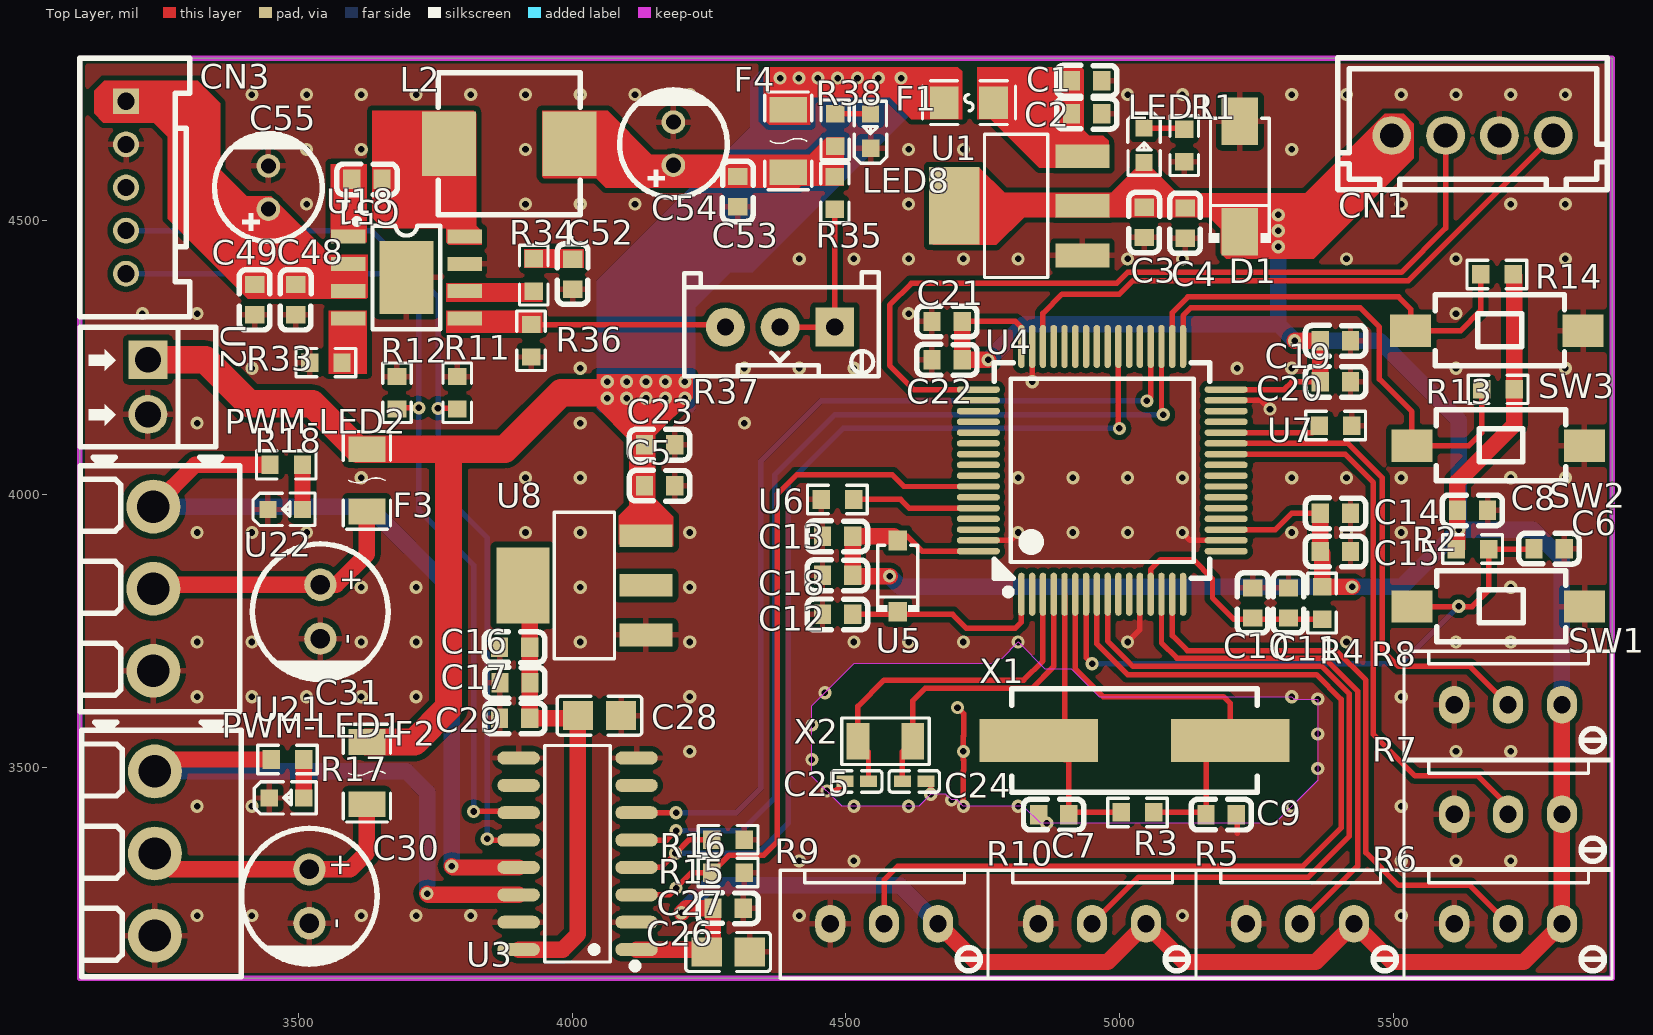
[diagram p0: Top Layer view]
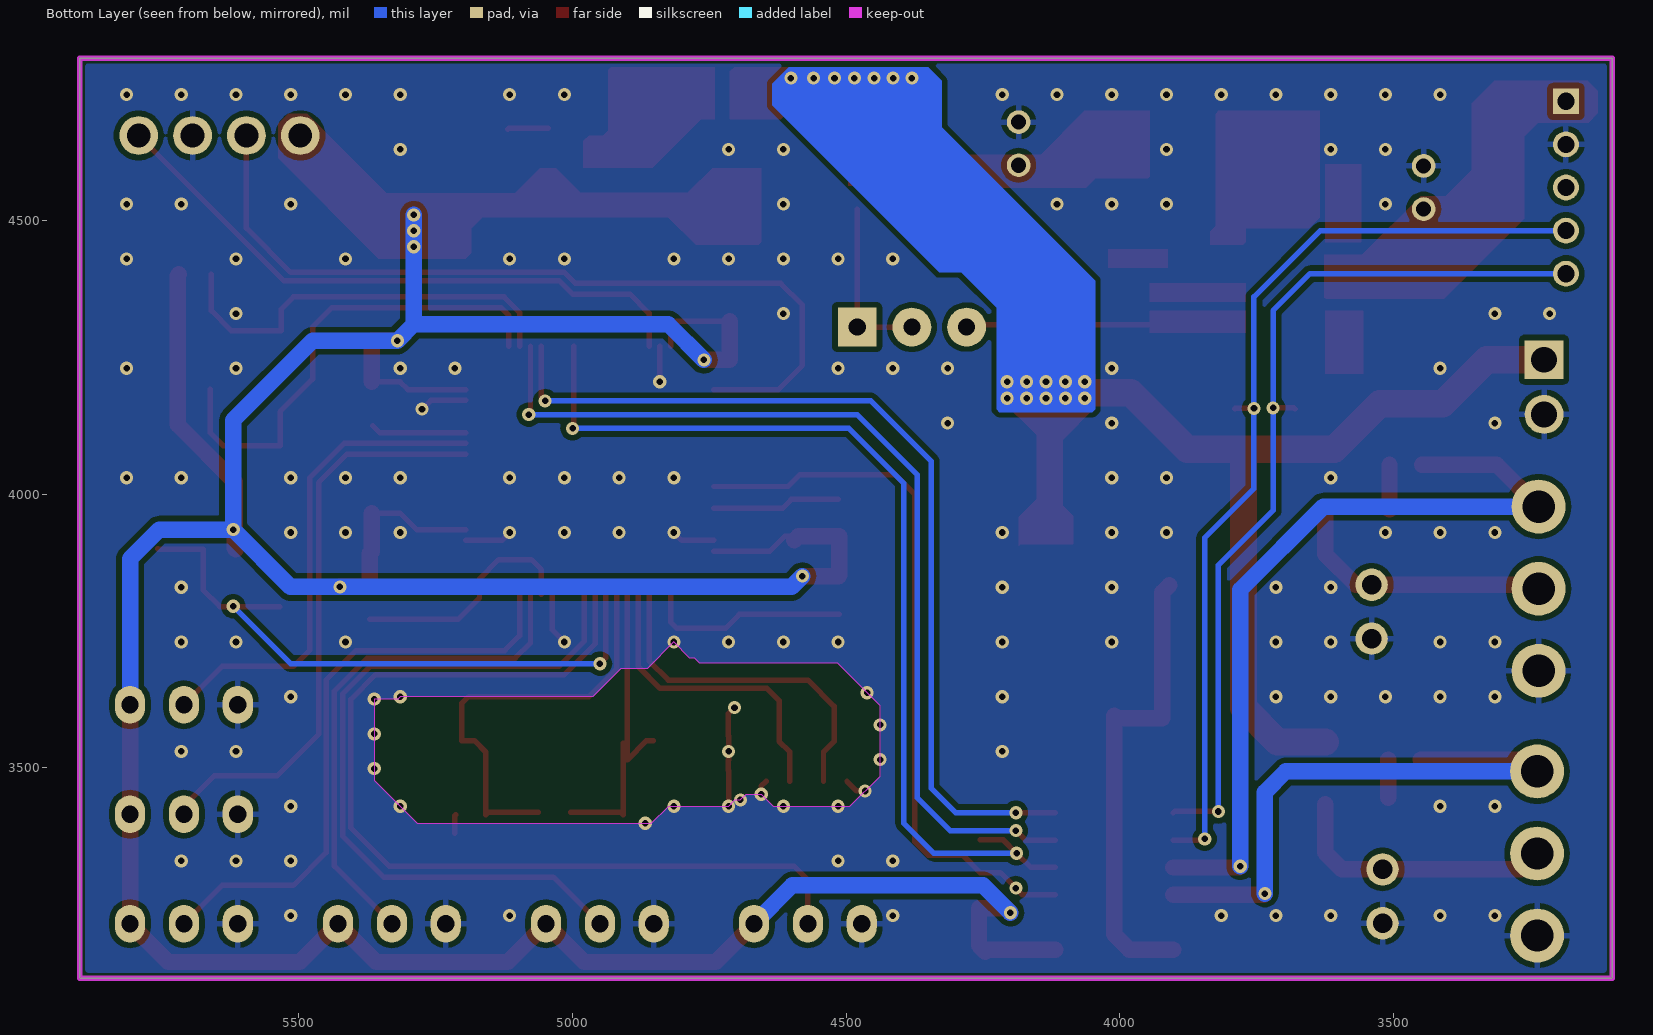
[diagram p1: Bottom Layer view, seen from below]
# Altium PCB MISC49876.pcbdoc
Units mil, origin at the board's own origin, x right, y up, seen from the top; angles counter-clockwise.
Board outline 2799.25 x 1680.67 mil, 2 copper layers (Top Layer, Bottom Layer), stack 62.206 mil thick; 90 components, 54 nets, 281 pads, 188 vias.

## Layer stack, top to bottom
Top Solder Mask Layer: solder mask 0.394, Dk 3.3
Top Layer: signal copper 1.379
Dielectric1: surface 59.449, FR4, Dk 4.5
Bottom Layer: signal copper 1.378
Bottom Solder Mask Layer: solder mask 0.394, Dk 3.3

## Board outline
3100.75,4796.22 3100.75,3115.55 5900,3115.55 5900,4796.22

## Design rules (kind name [scope] priority, off if disabled: settings)
BoardOutlineClearance copperThickness2oz_1 [All] p2 off: genericclearance=7.99 ignorepadtopadclearanceinfootprint=FALSE except(0: Arc-SplitContinuation Track-SplitContinuation SMDPad-SplitContinuation THPad-SplitContinuation Via-SplitContinuation Fill-SplitContinuation Region-SplitContinuation Poly-SplitContinuation Text-SplitContinuation Hole-SplitContinuation; 5.98: Arc-CutoutEdge SMDPad-CutoutEdge THPad-CutoutEdge Via-CutoutEdge Fill-CutoutEdge Region-CutoutEdge Text-CutoutEdge; 6.93: Hole-OutlineEdge Hole-CutoutEdge; 10: Poly-OutlineEdge Poly-CutoutEdge; 11.81: Arc-OutlineEdge Track-OutlineEdge SMDPad-OutlineEdge THPad-OutlineEdge Via-OutlineEdge Fill-OutlineEdge Region-OutlineEdge Text-OutlineEdge Track-CutoutEdge)
BoardOutlineClearance copperThickness1oz_1 [All] p4: genericclearance=4.02 ignorepadtopadclearanceinfootprint=FALSE except(0: Arc-SplitContinuation Track-SplitContinuation SMDPad-SplitContinuation THPad-SplitContinuation Via-SplitContinuation Fill-SplitContinuation Region-SplitContinuation Poly-SplitContinuation Text-SplitContinuation Hole-SplitContinuation; 6: SMDPad-CutoutEdge THPad-CutoutEdge Via-CutoutEdge Fill-CutoutEdge Region-CutoutEdge Text-CutoutEdge; 6.93: Hole-OutlineEdge Hole-CutoutEdge; 10: Poly-OutlineEdge Poly-CutoutEdge; 11.8: Arc-OutlineEdge Track-OutlineEdge SMDPad-OutlineEdge THPad-OutlineEdge Via-OutlineEdge Fill-OutlineEdge Region-OutlineEdge Text-OutlineEdge; 11.81: Arc-CutoutEdge Track-CutoutEdge)
Clearance copperThickness2oz [All] p1 off: gap=7.99 ignorepadtopadclearanceinfootprint=FALSE except(5.98: SMDPad-Track SMDPad-SMDPad THPad-Track SMDPad-THPad THPad-THPad Track-Via SMDPad-Via THPad-Via Via-Via Fill-Track Region-Track Fill-SMDPad Region-SMDPad Fill-THPad Region-THPad Fill-Via Region-Via Fill-Fill Fill-Region Region-Region Arc-Track Arc-SMDPad Arc-THPad Arc-Via Fill-Arc Region-Arc Arc-Arc Text-Track SMDPad-Text Text-THPad Text-Via Fill-Text Region-Text Arc-Text Text-Text; 6.93: Hole-Track Hole-SMDPad Hole-THPad Hole-Via Fill-Hole Region-Hole Hole-Arc Hole-Text; 10: Poly-Track Poly-SMDPad Poly-THPad Poly-Via Poly-Fill Poly-Region Poly-Poly Poly-Arc Poly-Text Poly-Hole)
Clearance copperThickness1oz [All] p3: gap=4.02 ignorepadtopadclearanceinfootprint=FALSE except(5.98: SMDPad-Track SMDPad-SMDPad THPad-Track SMDPad-THPad THPad-THPad Track-Via SMDPad-Via THPad-Via Via-Via Fill-Track Region-Track Fill-SMDPad Region-SMDPad Fill-THPad Region-THPad Fill-Via Region-Via Fill-Fill Fill-Region Region-Region; 6: Arc-Track Arc-SMDPad Arc-THPad Arc-Via Fill-Arc Region-Arc Arc-Arc Text-Track SMDPad-Text Text-THPad Text-Via Fill-Text Region-Text Arc-Text Text-Text; 6.93: Hole-Track Hole-SMDPad Hole-THPad Hole-Via Fill-Hole Region-Hole Hole-Arc Hole-Text; 10: Poly-Track Poly-SMDPad Poly-THPad Poly-Via Poly-Fill Poly-Region Poly-Poly Poly-Arc Poly-Text Poly-Hole)
DiffPairsRouting differentialPair [All] p1: maxlimit=6 minlimit=6 mostfreqgap=6 toplayer_minwidth=5 toplayer_prefwidth=10 toplayer_maxwidth=100 toplayer_mingap=6 toplayer_prefgap=6 toplayer_maxgap=6 bottomlayer_minwidth=5 bottomlayer_prefwidth=10 bottomlayer_maxwidth=100 bottomlayer_mingap=6 bottomlayer_prefgap=6 bottomlayer_maxgap=6 maxuncoupledlength=10
HoleToHoleClearance otherClearance [All] p1: gap=11.81 allowstackedmicrovias=TRUE
Length netLength [All] p1: minlimit=0 maxlimit=0
MatchedLengths netLengthTolerance [All] p1: tolerance=1000
PasteMaskExpansion pasteMaskExpansion [All] p1: expansion=0
PlaneConnect innerPlane [All] p1: planeconnectstyle=Relief reliefexpansion=20 reliefentries=4 reliefconductorwidth=10 reliefairgap=10
PolygonConnect copperRegion [(InNet('GND'))] p1: connectstyle=Relief reliefconductorwidth=10 reliefentries=4 polygonreliefangle="90 Angle" airgapwidth=10 via.connectstyle=Relief via.reliefconductorwidth=10 via.reliefentries=4 via.polygonreliefangle="90 Angle" via.airgapwidth=10
RoutingVias viaSize [All] p1: holewidth=12.01 width=24.02 viastyle="Through Hole" minholewidth=11.81 minwidth=19.68 maxholewidth=248.03 maxwidth=393.7
SolderMaskExpansion solderMaskExpansion [IsVia] p1: expansion=-1000 istentingtop=TRUE
SolderMaskExpansion solderMaskExpansion [All] p2: expansion=2 istentingtop=FALSE
Width copperThickness2oz_2 [All] p1 off: maxlimit=100 minlimit=8 preferedwidth=10
Width copperThickness1oz_2 [All] p2: maxlimit=100 minlimit=5 preferedwidth=10

## Components (designator, comment, footprint, x,y, rotation, side; value= is the part's Value field where it differs from the comment)
C1 "22uF" C0603 4940,4755 r180 top
C2 "100nF" C0603 4940,4695 r180 top
C3 "22uF" C0603 5045.23,4496.42 r90 top
C4 "100nF" C0603 5120,4495 r90 top
C5 "100nF" C0603 4160,4015 r0 top
C6 "100nF" C0603 5785,3900 r0 top
C7 "20pF" C0603 4880,3414.11 r0 top
C8 "100nF" C0603 5645,3970 r0 top
C9 "20pF" C0603 5185.77,3414.33 r180 top
C10 "100nF" C0603 5243.29,3800.87 r270 top
C11 "22uF" C0603 5308.85,3800.87 r270 top
C12 "100nF" C0603 4485,3780 r0 top
C13 "100nF" C0603 4485,3922.63 r0 top
C14 "100nF" C0603 5394.57,3964.89 r180 top
C15 "100nF" C0603 5394.57,3894.89 r180 top
C16 "22uF" C0603 3895,3720 r0 top
C17 "100nF" C0603 3895.61,3654.89 r0 top
C18 "100nF" C0603 4485,3851.32 r0 top
C19 "100nF" C0603 5394.57,4280 r180 top
C20 "100nF" C0603 5394.57,4205 r180 top
C21 "100nF" C0603 4685.01,4315.28 r0 top
C22 "100nF" C0603 4685.01,4245.02 r0 top
C23 "22uF" C0603 4160,4090 r0 top
C24 "9pF" C0402 4625,3475 r180 top
C25 "9pF" C0402 4520,3475 r0 top
C26 "10uF" C0805 4285,3163.34 r0 top
C27 "100nF" C0603 4285,3243.34 r180 top
C28 "10uF" C0805 4050,3595 r180 top
C29 "100nF" C0603 3895,3590 r180 top
C30 "1000uF" CAP-TH_BD6.3-P2.50-D0.5-FD 3520,3265 r270 top
C31 "1000uF" CAP-TH_BD6.3-P2.50-D0.5-FD 3540,3785 r270 top
C48 "100nF" C0603 3495,4355 r90 top
C49 "4.7uF" C0603 3420,4355 r90 top
C51 "100nF" C0603 3625,4575 r180 top
C52 "4.7nF" C0603 4000.83,4401.52 r270 top
C53 "47uF" C0603 4302.56,4552.56 r270 top
C54 "100uF" CAP-TH_BD5.0-P2.00-D0.5-FD 4185,4640 r90 top
C55 "100uF" CAP-TH_BD5.0-P2.00-D0.5-FD 3445,4560 r90 top
CN1 "HX25003-4A" CONN-TH_4P-P2.50_HX25003-4A 5645,4655 r180 top
CN3 "ZX-HY2.0-5PZZ" CONN-TH_5P-P2.00_ZX-HY2.0-5PZZ 3185,4560 r90 top
D1 "SS14" SMA_L4.2-W2.6-LS5.3-RD 5220,4580 r90 top
F1 "PICOSMDC050S-2" F0805 4725,4715 r0 top
F2 "JK-nSMD050-30" F1206 3625,3490 r90 top
F3 "JK-nSMD050-30" F1206 3625,4025 r90 top
F4 "SMD1206-050-16" F1206 4395,4645 r90 top
L2 "4.7uH" "0630 TPC 7*7*3" 3885,4640 r0 top
LED1 "" LED_0603 5045,4635 r270 top
LED8 "" LED_0603 4545,4665 r90 top
PWM-LED1 "" LED_0603 3480,3445 r0 top
PWM-LED2 "" LED_0603 3477.71,3972.13 r0 top
R1 "1kΩ" R0603 5118.46,4636.6 r90 top
R2 "10kΩ" R0603 5645.15,3899.36 r0 top
R3 "1MΩ" R0603 5032.88,3418.27 r0 top
R4 "10Ω" R0603 5370.26,3800.57 r270 top
R5 "5kΩ" RES-ADJ-TH_3296W-1-203 5330,3215 r0 top
R6 "5kΩ" RES-ADJ-TH_3296W-1-203 5710,3215 r0 top
R7 "5kΩ" RES-ADJ-TH_3296W-1-203 5710,3415 r0 top
R8 "5kΩ" RES-ADJ-TH_3296W-1-203 5710,3615 r0 top
R9 "5kΩ" RES-ADJ-TH_3296W-1-203 4570,3215 r0 top
R10 "5kΩ" RES-ADJ-TH_3296W-1-203 4950,3215 r0 top
R11 "10kΩ" R0603 3790,4185 r270 top
R12 "10kΩ" R0603 3680,4185 r270 top
R13 "10kΩ" R0603 5691.77,4191.18 r180 top
R14 "10kΩ" R0603 5689.56,4401.18 r180 top
R15 "10kΩ" R0603 4285,3308.34 r180 top
R16 "10kΩ" R0603 4285,3368.34 r180 top
R17 "1kΩ" R0603 3480,3515 r180 top
R18 "1kΩ" R0603 3477.71,4053.27 r180 top
R33 "200K" R0603 3550,4240 r0 top
R34 "20K" R0603 3930,4400 r90 top
R35 "27k" R0603 4480,4550 r90 top
R36 "8.2K" R0603 3925,4280 r90 top
R37 "50K" RESPOT3296 4380,4305 r180 top
R38 "1k" R0603 4480.53,4665.27 r270 top
SW1 "TS-1101-C-W" SW-SMD_L6.0-W3.3-LS8.0 5692.25,3794.36 r180 top
SW2 "TS-1101-C-W" SW-SMD_L6.0-W3.3-LS8.0 5691.77,4088.23 r180 top
SW3 "TS-1101-C-W" SW-SMD_L6.0-W3.3-LS8.0 5689.56,4298.23 r180 top
U1 "AMS1117-3.3" SOT-223-3_L6.5-W3.4-P2.30-LS7.0-BR 4815.23,4526.42 r0 top
U2 "DB125-2.54-2P-GN-S" CONN-TH_DB125-2.54-2P-GN 3225,4195.4 r270 top
U3 "π142U31" SOIC-16_L9.9-W3.9-P1.27-LS6.0-BL 4009.95,3342.69 r90 top
U4 "STM32F103RET6" LQFP-64_L10.0-W10.0-P0.50-LS12.0-BL 4968.51,4043.25 r0 top
U5 "IN4148 SMD diode" SOD-123_L2.7-W1.7-LS3.8-RD 4595,3850 r90 top
U6 "100k" R0603 4484.69,3990 r180 top
U7 "100k" R0603 5395,4125 r180 top
U8 "AMS1117-5.0" SOT-223_L6.5-W3.5-P2.30-LS7.0-BR 4022.43,3833.02 r0 top
U18 "SCT2450" SOP-8E 3697.19,4395.61 r0 top
U21 "DB125-3.81-3P-GN-S" CONN-TH_3P-P3.81_L7.4-W11.4 3237.71,3343.27 r270 top
U22 "DB125-3.81-3P-GN-S" CONN-TH_3P-P3.81_L7.4-W11.4 3235,3827.01 r270 top
X1 "8MHz" CRYSTAL-SMD_L11.5-W4.8-LS12.7 5027.4,3549.33 r0 top
X2 "32.768kHz" OSC-SMD_L3.2-W1.5 4572.4,3548.25 r0 top

## Footprints (in the part's own frame and the unit in brackets; to place one, negate y for a bottom-side part, rotate by r counter-clockwise, add the part's x,y. Pads: shape width x height; smd on the part's side, far side on the other; paste and mask are expansions set on the pad)
"0630 TPC 7*7*3" [mm]
  rect 2.5x3 smd: 1(-2.8,0) 2(2.8,0)
  silkscreen extent -3.3,-3.3 3.3,3.3
C0402 [mm]
  rect 0.79x0.54 smd paste-100 mask+0.051: 1(-0.545,0) 2(0.545,0)
  silkscreen extent -1.17,-0.5 1.17,0.5
C0603 [mm]
  rect 0.8x0.9 smd: 1(-0.7,0) 2(0.7,0)
  silkscreen extent -1.41,-0.71 1.39,0.72
C0805 [mm]
  rect 1.41x1.35 smd paste-100 mask+0.051: 1(-1,0) 2(1,0)
  silkscreen extent -1.96,-0.9 1.96,0.9
CAP-TH_BD5.0-P2.00-D0.5-FD [mm]
  round 1.1 hole 0.7 paste+0 mask+0.05: 1(-1,0) 2(1,0)
  silkscreen extent -2.5,-2.5 2.5,2.5
CAP-TH_BD6.3-P2.50-D0.5-FD [mm]
  round 1.5 hole 0.9 paste+0 mask+0.05: 1(-1.25,0) 2(1.25,0)
  silkscreen extent -3.15,-3.15 3.21,3.15
CONN-TH_3P-P3.81_L7.4-W11.4 [mm]
  round 2.5 hole 1.5: 1(-3.81,0) 2(0,0) 3(3.81,0)
  silkscreen extent -6.1,-3.4 5.71,4
CONN-TH_4P-P2.50_HX25003-4A [mm]
  round 1.8 hole 1.1: 1(-3.75,0) 2(-1.25,0) 3(1.25,0) 4(3.75,0)
  silkscreen extent -6.25,-3.6 6.25,2.51
CONN-TH_5P-P2.00_ZX-HY2.0-5PZZ [mm]
  rect 1.2x1.2 hole 0.8: 1(4,0)
  round 1.2 hole 0.8: 2(2,0) 3(0,0) 4(-2,0) 5(-4,0)
  silkscreen extent -6,-2.96 6,2.14
CONN-TH_DB125-2.54-2P-GN [mm]
  rect 1.8x1.8 hole 1.2: 1(-1.27,0)
  round 1.8 hole 1.2: 2(1.27,0)
  silkscreen extent -2.78,-3.14 2.78,3.14
CRYSTAL-SMD_L11.5-W4.8-LS12.7 [mm]
  rect 5.5x2 smd: 1(-4.45,0) 2(4.45,0)
  silkscreen extent -5.7,-2.4 5.7,2.4
F0805 [mm]
  rect 1.335x1.5 smd paste-100 mask+0.051: 1(-1.142,0) 2(1.142,0)
  silkscreen extent -2.16,-1.02 2.16,1.02
F1206 [mm]
  rect 1.19x1.728 smd: 1(-1.445,0) 2(1.445,0)
  silkscreen extent -2.27,-1.09 2.27,1.09
LED_0603 [mil]
  rect 31.5x31.5 smd paste+0 mask+2: 1(-33.5,-0.4) 2(29.5,-0.2)
  silkscreen extent -61,-30 53,30
LQFP-64_L10.0-W10.0-P0.50-LS12.0-BL [mm]
  oval 0.3x2 smd: 1(-3.75,-5.75) 2(-3.25,-5.75) 3(-2.75,-5.75) 4(-2.25,-5.75) 5(-1.75,-5.75) 6(-1.25,-5.75) 7(-0.75,-5.75) 8(-0.25,-5.75) 9(0.25,-5.75) 10(0.75,-5.75) 11(1.25,-5.75) 12(1.75,-5.75) 13(2.25,-5.75) 14(2.75,-5.75) 15(3.25,-5.75) 16(3.75,-5.75) 33(3.75,5.75) 34(3.25,5.75) 35(2.75,5.75) 36(2.25,5.75) 37(1.75,5.75) 38(1.25,5.75) 39(0.75,5.75) 40(0.25,5.75) 41(-0.25,5.75) 42(-0.75,5.75) 43(-1.25,5.75) 44(-1.75,5.75) 45(-2.25,5.75) 46(-2.75,5.75) 47(-3.25,5.75) 48(-3.75,5.75)
  oval 2x0.3 smd: 17(5.75,-3.75) 18(5.75,-3.25) 19(5.75,-2.75) 20(5.75,-2.25) 21(5.75,-1.75) 22(5.75,-1.25) 23(5.75,-0.75) 24(5.75,-0.25) 25(5.75,0.25) 26(5.75,0.75) 27(5.75,1.25) 28(5.75,1.75) 29(5.75,2.25) 30(5.75,2.75) 31(5.75,3.25) 32(5.75,3.75) 49(-5.75,3.75) 50(-5.75,3.25) 51(-5.75,2.75) 52(-5.75,2.25) 53(-5.75,1.75) 54(-5.75,1.25) 55(-5.75,0.75) 56(-5.75,0.25) 57(-5.75,-0.25) 58(-5.75,-0.75) 59(-5.75,-1.25) 60(-5.75,-1.75) 61(-5.75,-2.25) 62(-5.75,-2.75) 63(-5.75,-3.25) 64(-5.75,-3.75)
  silkscreen extent -5,-5.79 5,5
OSC-SMD_L3.2-W1.5 [mm]
  rect 1.05x1.7 smd: 1(-1.275,0) 2(1.275,0)
  silkscreen extent -2.03,-1.08 2.03,1.08
R0603 [mil]
  rect 31.75x34.02 smd paste-3937.01 mask+2: 1(-29.66,0) 2(29.66,0)
  silkscreen extent -55,-26 55,26
RES-ADJ-TH_3296W-1-203 [mm]
  oval 1.4x1.75 hole 0.8: 1(-2.5,0) 2(0,0) 3(2.5,0)
  silkscreen extent -4.83,-2.53 4.83,2.48
RESPOT3296 [mm]
  rect 1.8x1.8 hole 0.8: 1(-2.54,0)
  round 1.8 hole 0.8: 2(2.54,0) ADJ(0,0)
  silkscreen extent -4.57,-2.54 4.44,2.29
SMA_L4.2-W2.6-LS5.3-RD [mm]
  rect 2.2x1.7 smd: 1(-2.565,0) 2(2.565,0)
  silkscreen extent -3.08,-1.44 2.7,1.44
SOD-123_L2.7-W1.7-LS3.8-RD [mm]
  rect 0.91x0.84 smd: 1(-1.655,0) 2(1.655,0)
  silkscreen extent -1.65,-1 1.43,1
SOIC-16_L9.9-W3.9-P1.27-LS6.0-BL [mil]
  oval 23.7x77.6 smd: 1(-175,-107.7) 2(-125,-107.7) 3(-75,-107.7) 4(-25,-107.7) 5(25,-107.7) 6(75,-107.7) 7(125,-107.7) 8(175,-107.7) 9(175,107.7) 10(125,107.7) 11(75,107.7) 12(25,107.7) 13(-25,107.7) 14(-75,107.7) 15(-125,107.7) 16(-175,107.7)
  silkscreen extent -211,-111 198,60
SOP-8E [mm]
  rect 2.5x3.4 smd: 0(0,0)
  rect 1.6x0.65 smd: 1(-2.7,1.905) 2(-2.7,0.635) 3(-2.7,-0.635) 4(-2.7,-1.905) 5(2.7,-1.905) 6(2.7,-0.635) 7(2.7,0.635) 8(2.7,1.905)
  silkscreen extent -2.42,-2.4 1.58,2.72
SOT-223-3_L6.5-W3.4-P2.30-LS7.0-BR [mm]
  rect 2.5x1.1 smd: 1(2.97,-2.3) 2(2.97,0) 3(2.97,2.3)
  rect 2.34x3.6 smd: 4(-2.97,0)
  silkscreen extent -1.57,-3.33 1.37,3.33
SOT-223_L6.5-W3.5-P2.30-LS7.0-BR [mm]
  rect 2.465x1.05 smd: 1(2.857,-2.3) 2(2.857,0) 3(2.857,2.3)
  rect 2.465x3.54 smd: 4(-2.857,0)
  silkscreen extent -1.4,-3.4 1.4,3.4
SW-SMD_L6.0-W3.3-LS8.0 [mm]
  rect 1.9x1.5 smd: 1(-4,0) 2(4,0)
  silkscreen extent -3.14,-1.67 2.86,1.63

## Via types
v1: diameter 24.02, hole 12, Top Layer to Bottom Layer, 188 vias

## Nets (pads, with @x,y where several pads share a name; then routed paths per layer and width w, separated by ;. In a path a pad name is that pad's centre, name@x,y a point inside that pad or via, vN(x,y) a via of type N, cw(c..) or ccw(c..) an arc to the next point about the centre after c; other vN are vias at no path point)
3V3: C3.2 C4.2 C8.1 C13.2 C14.2 C15.2 C18.2 C19.2 C20.2 C21.2 C22.2 C26.1 C27.2 CN1.4 D1.1 LED1.2 R2.1 R4.1 R5.3 R6.3 R7.3 R8.3 R9.3 R10.3 R13.1 R14.1 U1.2 U1.4 U3.1 U4.19 U4.32 U4.48 U4.64 U5.2 | length 7313.4
  Top Layer w10: U5.2@4587.53,3922.63 4612.37,3922.63 4639.39,3895.61 U4.64 ; C21.2 4809.72,4315.28 4820.87,4304.13 U4.48 ; U4.19 5284.98,3934.98 5314.89,3964.89 C14.2 ; U4.32 5300.89,4190.89 5315,4205 C20.2
  Top Layer w30: U3.1 4241.28,3167.69 C26.1 4257.44,3175.15 C27.2 4208.34,3243.34 v1(4200,3235) ; v1(4580,3850) 4513.88,3850 C18.2 C13.2 4587.53,3922.63 U5.2 ; R9.3 4738.43,3145 4978.42,3145 R10.3 5118.43,3145 5358.42,3145 R5.3 5498.43,3145 5738.42,3145 R6.3 R7.3 R8.3 ; C22.2 C21.2 ; C22.2 v1(4760,4245) ; v1(5320,4280) C19.2 C20.2 ; C14.2 C15.2 5370.26,3891.64 R4.1 v1(5425,3830.23) ; R2.1 5617.44,3901.31 C8.1 5617.44,4022.44 5721.43,4126.43 R13.1 5721.43,4398.98 R14.1
  Bottom Layer w30: v1(4200,3235) 4250,3285 4598.43,3285 R9.3 ; v1(4580,3850) 4599.77,3830.23 v1(5425,3830.23) 5515.23,3830.23 v1(5620,3935) ; v1(4760,4245) 4825,4310 5290,4310 ; v1(5290,4510) v1(5290,4481.01) v1(5290,4451.75) 5290,4310 ; R8.3 5808.42,3881.58 5755,3935 v1(5620,3935) ; 5290,4310 v1(5320,4280) 5475,4280 5620,4135 v1(5620,3935)
$1N875: C1.2 C2.2 F1.2 U1.3
$1N876: LED1.1 R1.2 | length 74.8
  Top Layer w10: LED1.1 5116.22,4668.5 R1.2
$1N10668: R33.2 U18.4
$1N12142: C51.2 U18.1
$1N12147: C51.1 L2.1 U18.8
$1N12206: C52.1 R34.2
$1N12210: R34.1 U18.6
$1N12341: C53.1 C54.1 F4.1 L2.2 R35.2 R38.2
$1N12507: R35.1 R37.1 R37.ADJ | length 315.3
  Top Layer w10: R37.ADJ R37.1 R35.1
$1N12535: R36.2 R37.2 U18.5 | length 356.9
  Top Layer w10: R36.2 4275.34,4309.66 R37.2
$1N12695: LED8.2 R38.1 | length 64.8
  Top Layer w10: R38.1 4544.77,4694.93 LED8.2
$2N480: C24.2 U4.4 X2.2 | length 570.6
  Top Layer w10: C24.2 4603.54,3529.18 X2.2 4622.6,3622.6 4645,3645 4840,3645 4879.93,3684.93 U4.4
$2N481: C25.2 U4.3 X2.1 | length 639.2
  Top Layer w10: C25.2 4541.46,3528.99 X2.1 4522.2,3612.2 4570,3660 4825,3660 4860.24,3695.24 U4.3
$2N849: C7.2 R3.1 U4.5 X1.1 | length 603.3
  Top Layer w10: X1.1 4865,3549.33 X1.1@4900,3514.33 ; U4.5 4900,3816.49 X1.1@4900,3514.33 ; X1.1@4907.56,3544.33 X1.1@4907.56,3521.89 ; R3.1 4911.72,3418.27 C7.2 X1.1@4907.56,3521.89 ; X1.1@4900,3514.33 X1.1@4907.56,3521.89
$2N857: C9.2 R3.2 U4.6 X1.2 | length 778.1
  Top Layer w10: U4.6 4919.3,3680.7 4970,3630 5190,3630 5202.6,3617.4 X1.2 5179.33,3549.33 5158.21,3528.21 C9.2 5154.26,3418.27 R3.2
$2N1069: U4.60 U6.1 | length 234.3
  Top Layer w10: U6.1 4600,3990 4615.65,3974.35 U4.60
$4N719: C30.1 F2.1 U21.2 | length 500.2
  Top Layer w30: U21.2 3266.77,3314.21 C30.1 3594.21,3314.21 3625,3345 F2.1
$4N967: PWM-LED1.2 R17.1 | length 70.3
  Top Layer w30: PWM-LED1.2 3509.66,3444.96 R17.1
$4N1198: C31.1 F3.1 U22.2 | length 494.2
  Top Layer w30: U22.2 3242.2,3834.21 C31.1 3569.21,3834.21 3625,3890 F3.1
$4N1205: PWM-LED2.2 R18.1 | length 81.4
  Top Layer w30: PWM-LED2.2 3507.37,3972.09 R18.1
+5V: C16.2 C17.2 C28.2 C29.1 U3.16 U8.4 | length 857.7
  Top Layer w30: U3.16 3982.69,3167.69 4010.63,3195.63 C28.2 4005.63,3590 C29.1 C16.2 3922.56,3820.39 U8.4
+6V: C5.1 C23.1 F1.1 F2.2 F3.2 F4.2 U2.1 U8.3 | length 1623.1
  Top Layer w50: U2.1 3329.6,4245.4 3410,4165 3525,4165 3608.11,4081.89 F3.2 3774.09,4081.89 ; F2.2 3711.89,3546.89 3774.09,3609.09 3774.09,4081.89 ; 4090,4185 3980,4185 3876.89,4081.89 3774.09,4081.89
  other v1: 4064.07,4175 4099.53,4175 4135,4175 4170.47,4175 4205.93,4175 4064.07,4205 4099.53,4205 4135,4205 4170.47,4205 4205.93,4205 4380,4760 4414.19,4760 4449.05,4760 4484.94,4760 4521.36,4760 4559.6,4760 4600.96,4760
ADBY1: R9.2 U4.8 | length 1768.2
  Top Layer w10: R9.2 4569.99,3294.99 4595,3320 5335,3320 5405,3390 5405,3625 5360,3670 5015,3670 4958.67,3726.33 U4.8
ADBY2: R10.2 U4.9 | length 1363.2
  Top Layer w10: R10.2 5034.99,3300 5345,3300 5420,3375 5420,3635 5370,3685 5025,3685 4978.35,3731.65 U4.9
ADCLOSESPEED: R8.2 U4.27 | length 897.4
  Top Layer w10: U4.27 5417.54,4092.46 5480,4030 5480,3715 5510,3685 5639.99,3685 R8.2
ADOPENSPEED: R7.2 U4.26 | length 1065.8
  Top Layer w10: U4.26 5412.22,4072.78 5464.02,4020.98 5464.02,3560.98 5540,3485 5655,3485 5709.99,3430.01 R7.2
ADSETCLOSE: R6.2 U4.15 | length 1091.5
  Top Layer w10: U4.15 5096.46,3741.46 5123.9,3714.02 5395.98,3714.02 5450,3660 5450,3345 5510,3285 5639.99,3285 R6.2
ADSETOPEN: R5.2 U4.14 | length 951.9
  Top Layer w10: U4.14 5076.78,3728.22 5105,3700 5375,3700 5435,3640 5435,3320.01 R5.2
BAT: C12.2 U4.1 U5.1 | length 374.2
  Top Layer w10: C12.2 4695,3780 4720,3755 4810,3755 4820.87,3765.87 U4.1
BOOT1: U4.28 U7.2 | length 175.8
  Top Layer w10: U4.28 5352.49,4112.15 U7.2
CLOSE_CONTROL: CN3.5 R12.2 U3.11 | length 1643.4
  Top Layer w10: R12.2 3682,4157.34 v1(3720,4157.34) ; v1(3820,3420) 3899.94,3420 U3.11
  Bottom Layer w10: CN3.5 3652.48,4402.52 3720,4335 v1(3720,4157.34) 3720,3970 3820,3870 v1(3820,3420)
CLOSE_TEST: R14.2 SW3.2 U4.34 | length 767.4
  Top Layer w10: U4.34 5096.46,4331.46 5125,4360 5510,4360 5532.08,4337.92 SW3.2 5623.23,4298.23 5659.9,4334.9 R14.2
DOOR_CLOSE: U3.6 U4.36 | length 1696.4
  Top Layer w10: U3.6 v1(4190,3417.69) ; v1(5050,4170) 5057.09,4177.09 U4.36
  Bottom Layer w10: v1(4190,3417.69) 4300,3417.69 4345,3462.69 4345,4060 4455,4170 v1(5050,4170)
DOOR_OPEN: U3.5 U4.35 | length 1755.9
  Top Layer w10: U3.5 4172.69,3367.69 v1(4190,3385) ; U4.35 5076.78,4148.22 v1(5080,4145)
  Bottom Layer w10: v1(4190,3385) 4310,3385 4370,3445 4370,4035 4480,4145 v1(5080,4145)
EHERNET_RST: U4.20
GD1: U4.21
GD2: U4.22
GND: C1.1 C2.1 C3.1 C4.1 C5.2 C6.2 C7.1 C8.2 C9.1 C10.1 C11.1 C12.1 C13.1 C14.1 C15.1 C16.1 C17.1 C18.1 C19.1 C20.1 C21.1 C22.1 C23.2 C24.1 C25.1 C26.2 C27.1 C28.1 C29.2 C30.2 C31.2 C48.1 C49.1 C52.2 C53.2 C54.2 C55.2 CN1.2 CN3.2 D1.2 LED8.1 PWM-LED1.1 PWM-LED2.1 R1.1 R5.1 R6.1 R7.1 R8.1 R9.1 R10.1 R11.1 R12.1 R15.1 R16.1 R33.1 R36.1 SW1.1 SW2.1 SW3.1 U1.1 U2.2 U3.2 U3.8 U3.9 U3.15 U4.12 U4.18 U4.31 U4.47 U4.63 U6.2 U7.1 U8.1 U18.0 U18.7 U21.3 U22.3 | length 701.2
  Top Layer w10: v1(4465.4,3457.43) 4480.97,3457.43 C25.1 ; C24.1 4655.27,3466.19 v1(4655.27,3451.4) ; v1(4704.04,3609.88) 4715.55,3598.37 4715.55,3558.27 4714.85,3557.57 v1(4714.85,3529.65) 4714.85,3514.63 4715.55,3513.93 4715.55,3494.89 4714.85,3494.18 v1(4714.85,3429.65) ; U4.63 4800.5,3915.3 v1(4814.85,3929.65) ; v1(4840.56,4205) U4.47 ; v1(5014.85,3729.65) 5037.41,3752.21 U4.12 ; v1(5114.85,3929.65) 5129.2,3915.3 U4.18 ; U4.31 5258.8,4171.2 v1(5275,4155) ; C9.1 5215,3412.66 5215,3380
  other v1: 3314.85,3229.65 3414.85,3229.65 3614.85,3229.65 3714.85,3229.65 3814.85,3229.65 4414.85,3229.65 5114.85,3229.65 5514.85,3229.65 4414.85,3329.65 4514.85,3329.65 5514.85,3329.65 5614.85,3329.65 5714.85,3329.65 4867.17,3398.46 3314.85,3429.65 3414.85,3429.65 4514.85,3429.65 4614.85,3429.65 4814.85,3429.65 5314.85,3429.65 5514.85,3429.65 4693.32,3441.03 5362.25,3498.42 4438.16,3514.66 4214.85,3529.65 5614.85,3529.65 5714.85,3529.65 5362.25,3561.8 4438.16,3578.05 5362.25,3625.19 3314.85,3629.65 3414.85,3629.65 3514.85,3629.65 3614.85,3629.65 3714.85,3629.65 4214.85,3629.65 5314.85,3629.65 5514.85,3629.65 4461.7,3636.9 3314.85,3729.65 3414.85,3729.65 3614.85,3729.65 3714.85,3729.65 4014.85,3729.65 4214.85,3729.65 4514.85,3729.65 4614.85,3729.65 4714.85,3729.65 4814.85,3729.65 5414.85,3729.65 5614.85,3729.65 5714.85,3729.65 3614.85,3829.65 3714.85,3829.65 4014.85,3829.65 4214.85,3829.65 5714.85,3829.65 3314.85,3929.65 3414.85,3929.65 3514.85,3929.65 3914.85,3929.65 4014.85,3929.65 4214.85,3929.65 4914.85,3929.65 5014.85,3929.65 5314.85,3929.65 5414.85,3929.65 5514.85,3929.65 3614.85,4029.65 3914.85,4029.65 4014.85,4029.65 4814.85,4029.65 4914.85,4029.65 5014.85,4029.65 5114.85,4029.65 5314.85,4029.65 5414.85,4029.65 5514.85,4029.65 5714.85,4029.65 5814.85,4029.65 3314.85,4129.65 4014.85,4129.65 4314.85,4129.65 3414.85,4229.65 4014.85,4229.65 4314.85,4229.65 4414.85,4229.65 4514.85,4229.65 5214.85,4229.65 5314.85,4229.65 5614.85,4229.65 5814.85,4229.65 3214.85,4329.65 3314.85,4329.65 4614.85,4329.65 5614.85,4329.65 4414.85,4429.65 4514.85,4429.65 4614.85,4429.65 4714.85,4429.65 4814.85,4429.65 5014.85,4429.65 5114.85,4429.65 5414.85,4429.65 5614.85,4429.65 5814.85,4429.65 3514.85,4529.65 3914.85,4529.65 4014.85,4529.65 4114.85,4529.65 4614.85,4529.65 5514.85,4529.65 5714.85,4529.65 5814.85,4529.65 3514.85,4629.65 3614.85,4629.65 3914.85,4629.65 4614.85,4629.65 4714.85,4629.65 5314.85,4629.65 3414.85,4729.65 3514.85,4729.65 3614.85,4729.65 3714.85,4729.65 3814.85,4729.65 3914.85,4729.65 4014.85,4729.65 4114.85,4729.65 4214.85,4729.65 5014.85,4729.65 5114.85,4729.65 5314.85,4729.65 5414.85,4729.65 5514.85,4729.65 5614.85,4729.65 5714.85,4729.65 5814.85,4729.65
NRST: C6.1 R2.2 SW1.2 U4.7 | length 1155
  Top Layer w10: U4.7 4938.98,3701.02 v1(4950,3690) ; SW1.2 5644.36,3794.36 5674.81,3824.81 R2.2 5756.8,3899.36 C6.1
  Bottom Layer w10: v1(4950,3690) 5515,3690 v1(5620,3795)
OPEN_CONTROL: CN3.4 R11.2 U3.12 | length 1741.2
  Top Layer w10: v1(3755,4156.56) 3788.78,4156.56 R11.2 ; v1(3845,3370) 3847.31,3367.69 U3.12
  Bottom Layer w10: CN3.4 3633.74,4481.26 3755,4360 v1(3755,4156.56) 3755,4010 3845,3920 v1(3845,3370)
OPEN_TEST: R13.2 SW2.2 U4.33 | length 893.7
  Top Layer w10: U4.33 5116.15,4326.15 5130,4340 5440,4340 5475,4305 5475,4210 5534.29,4150.71 SW2.2 5638.23,4088.23 5662.11,4112.11 R13.2
PA2-TX: U4.16
PA3-RX: U4.17
PA13: CN1.1 U4.46 | length 1127.5
  Top Layer w10: U4.46 4860.24,4330.24 4895,4365 5000,4365 5025,4390 5527.64,4390 CN1.1
PA14: CN1.3 U4.49 | length 1533.7
  Top Layer w10: U4.49 4624.11,4190.89 4580,4235 4580,4345 4620,4385 4995,4385 5015,4405 5515,4405 5595.78,4485.78 CN1.3
PB6-PWM1: R15.2 U3.3 U4.58 | length 1323.1
  Top Layer w10: U3.3 4177.69,3267.69 v1(4190,3280) 4218.34,3308.34 R15.2 4287,3340 4350,3340 4375,3365 4375,4000 4410,4035 4585,4035 4606.28,4013.72 U4.58
PC8-PWM2: R16.2 U3.4 U4.39 | length 1806.2
  Top Layer w10: U3.4 4162.69,3317.69 v1(4188.55,3343.55) 4213.34,3368.34 R16.2 ; U4.39 4998.04,4121.96 v1(5000,4120)
  Bottom Layer w10: v1(4188.55,3343.55) 4340,3343.55 4395,3398.55 4395,4020 4495,4120 v1(5000,4120)
PWM1: R17.2 U3.14 U21.1 | length 1088
  Top Layer w30: U21.1 3259.44,3515 R17.2 ; v1(3735,3270) 3737.31,3267.69 U3.14
  Bottom Layer w30: U21.1 3696.73,3493.27 3735,3455 v1(3735,3270)
PWM2: R18.2 U3.13 U22.1 | length 1480.8
  Top Layer w30: U22.1 3311.26,4053.27 R18.2 ; v1(3780,3320) 3782.31,3317.69 U3.13
  Bottom Layer w30: U22.1 3627.99,3977.01 3780,3825 v1(3780,3320)
USART1_RX: U4.43
USART1_TX: U4.42
V24+: C48.2 C49.2 C55.1 CN3.1 U18.2 U18.3
VDDA: C10.2 C11.2 R4.2 U4.13 | length 431.5
  Top Layer w10: U4.13 5057.09,3862.09 5075,3880 5135,3880 5170,3845 5170,3810 5209.09,3770.91 R4.2
pads on no net: CN3.3 U3.7 U3.10 U4.2 U4.10 U4.11 U4.23 U4.24 U4.25 U4.29 U4.30 U4.37 U4.38 U4.40 U4.41 U4.44 U4.45 U4.50 U4.51 U4.52 U4.53 U4.54 U4.55 U4.56 U4.57 U4.59 U4.61 U4.62 U8.2

## Polygon pours and split planes (outlines as drawn)
GND on Top Layer (solid, remove dead copper, pour order 0): 3000,4880 3000,3000 5990,3000 5990,4880
GND on Bottom Layer (solid, remove dead copper, pour order 2): 3053.94,4860.16 3053.94,3035 5975,3035 5975,4860.16

## Keep-outs
Board Outline Layer:
  region: 4814.85,3729.65 4863.79,3680.7 4911.56,3680.7 4962.61,3629.65 5314.85,3629.65 5319.3,3625.19 5362.25,3625.19 5362.25,3477.05 5283.66,3398.46 4855.85,3398.46 4824.66,3429.65 4714.85,3429.65 4703.47,3441.03 4693.32,3441.03 4682.94,3451.4 4655.27,3451.4 4633.51,3429.65 4493.18,3429.65 4438.16,3484.67 4438.16,3613.35 4515.55,3690.74 4767.46,3690.74 4776.91,3700.19 4785.4,3700.19
  lines w10: 3100.75,3115.55 3100.75,4796.22 5900,4796.22 5900,3115.55 3100.75,3115.55

## Other copper
Top Layer:
  region net V24+: 3145,4755 3316.1,4755 3357,4714.1 3357,4592.6 3405.4,4544.2 3450.6,4544.2 3557.8,4437 3626.2,4437 3626.2,4358.9 3623.9,4356.6 3407.76,4356.6 3260.99,4503.37 3260.99,4653.11 3235.5,4678.6 3143.4,4678.6 3126.7,4695.3 3126.7,4736.7
  region net $1N10668: 3555,4335 3555,4220 3625,4220 3625,4335
  region net $1N12210: 3770,4385 3770,4350.98 3945.75,4350.98 3945.75,4385
  region net $1N12535: 3770,4335 3770,4295 3945,4295 3945,4335
  region net $1N12206: 3912.28,4447.05 3912.28,4413.16 4021.07,4413.16 4021.07,4447.05
  region net $1N12142: 3558.7,4602.72 3558.7,4460 3625,4460 3625,4602.72
  region net $1N12147: 3635,4700 3820,4700 3825,4695 3825,4490 3835,4480 3835,4455 3775,4455 3770,4460 3770,4485.86 3654.14,4485.86 3635,4505
  region net $1N12341: 3945,4700 4065,4700 4145,4620 4433.1,4620 4464.79,4651.69 4496.28,4651.69 4496.28,4563.58 4418.58,4563.58 4415,4560 4061.25,4560 4044.24,4577.01 3947.99,4577.01 3945,4580
  region net +6V: 4360,4675 4350,4685 4350,4780 4705,4780 4712.69,4772.31 4712.69,4685 4620,4685 4580,4725 4440,4725 4435,4720 4435,4675
  region net $1N875: 4740,4780 4930,4780 4935,4775 4935,4665 4945,4655 4970,4655 4980,4645 4980,4596.4 4853.6,4596.4 4765,4685 4740,4685
  region net +6V: 4045,4219.24 4219.41,4219.24 4220,4218.65 4220,4175 4152.32,4107.32 4152.32,3991.55 4185,3958.87 4185,3905 4182.13,3907.87 4085,3907.87 4085,3960 4104.67,3979.67 4104.67,4098.67 4045,4158.34
  region net 3V3: 5519.52,4695 5538.07,4676.46 5538.07,4613.07 5355,4430 5195,4430 5185,4440 5185,4485 5163.97,4506.03 4826.03,4506.03 4775,4455 4660,4455 4655,4460 4655,4595 4745,4595 4790,4550 4985,4550 5030,4595 5060,4595 5105.27,4549.73 5339.73,4549.73 5485,4695
Bottom Layer:
  region net +6V: 4350,4780 4605,4780 4635,4750 4635,4710 4330,4405 4290,4405 4225,4340 4225,4154.67 4220,4149.67 4050.33,4149.67 4045,4155 4045,4390 4325,4670 4325,4755